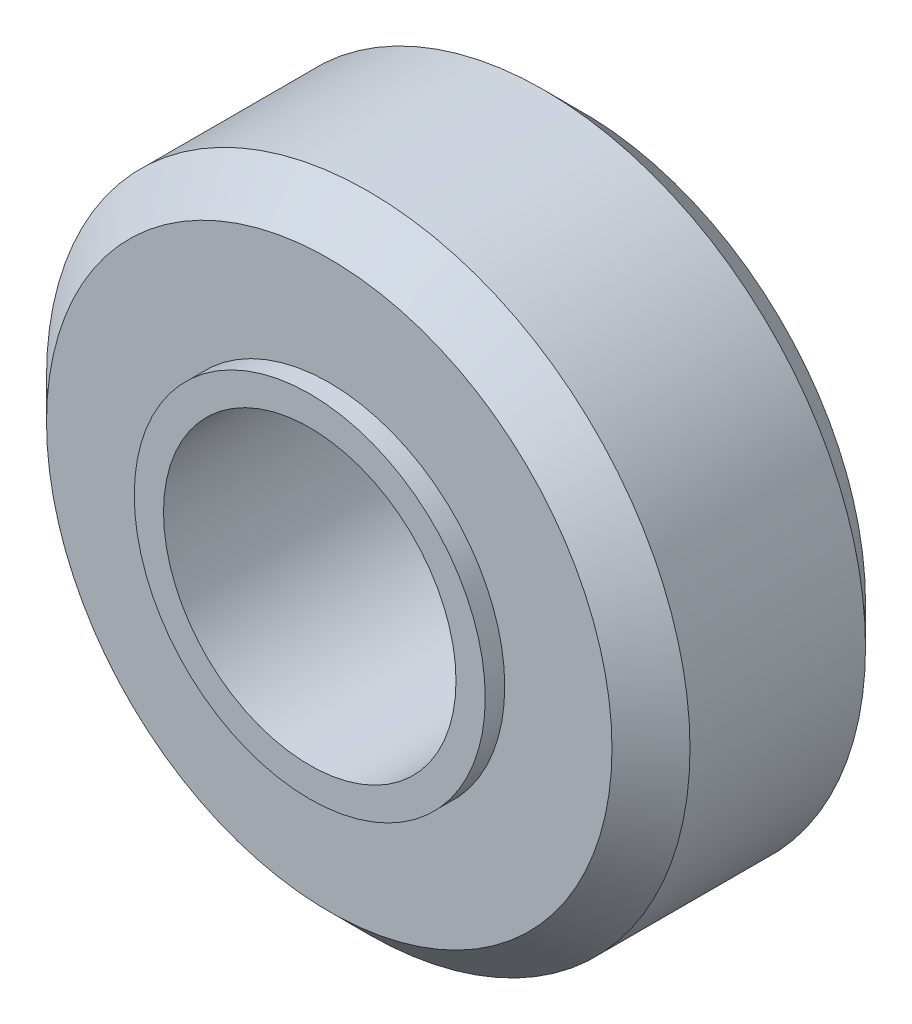
SolidWorks part; units mm, degrees
ref_plane "前视基准面" through (0, 0, 0) normal (0, 0, 1) x (1, 0, 0)
ref_plane "上视基准面" through (0, 0, 0) normal (0, 1, 0) x (1, 0, 0)
ref_plane "右视基准面" through (0, 0, 0) normal (1, 0, 0) x (0, 0, -1)
sketch "草图1" plane through (0, 0, 0) normal (0, 0, 1) x (1, 0, 0)
  circle A0 centre (0, 0) radius 7.5
  circle A1 centre (0, 0) radius 16.5
  dimension "D1" = 15
  dimension "D2" = 33
extrude "凸台-拉伸1" add sketch "草图1" along normal blind 10
sketch "草图2" plane through (0, 0, 10) normal (0, 0, 1) x (1, 0, 0)
  circle A0 centre (0, 0) radius 9
  circle A1 centre (0, 0) radius 7.5 construction
  circle A2 centre (0, 0) radius 7.5
  dimension "D1" = 18
extrude "凸台-拉伸2" add sketch "草图2" along normal blind 1
sketch "草图3" plane through (0, 0, 0) normal (0, 0, -1) x (-1, 0, 0)
  circle A0 centre (0, 0) radius 16.5 construction
  circle A1 centre (0, 0) radius 16.5
extrude "凸台-拉伸3" add sketch "草图3" along normal blind 3
chamfer "倒角1" distance 2 angle 45 2 edges at (16.5, 0, 10) (-16.5, 0, -3)
